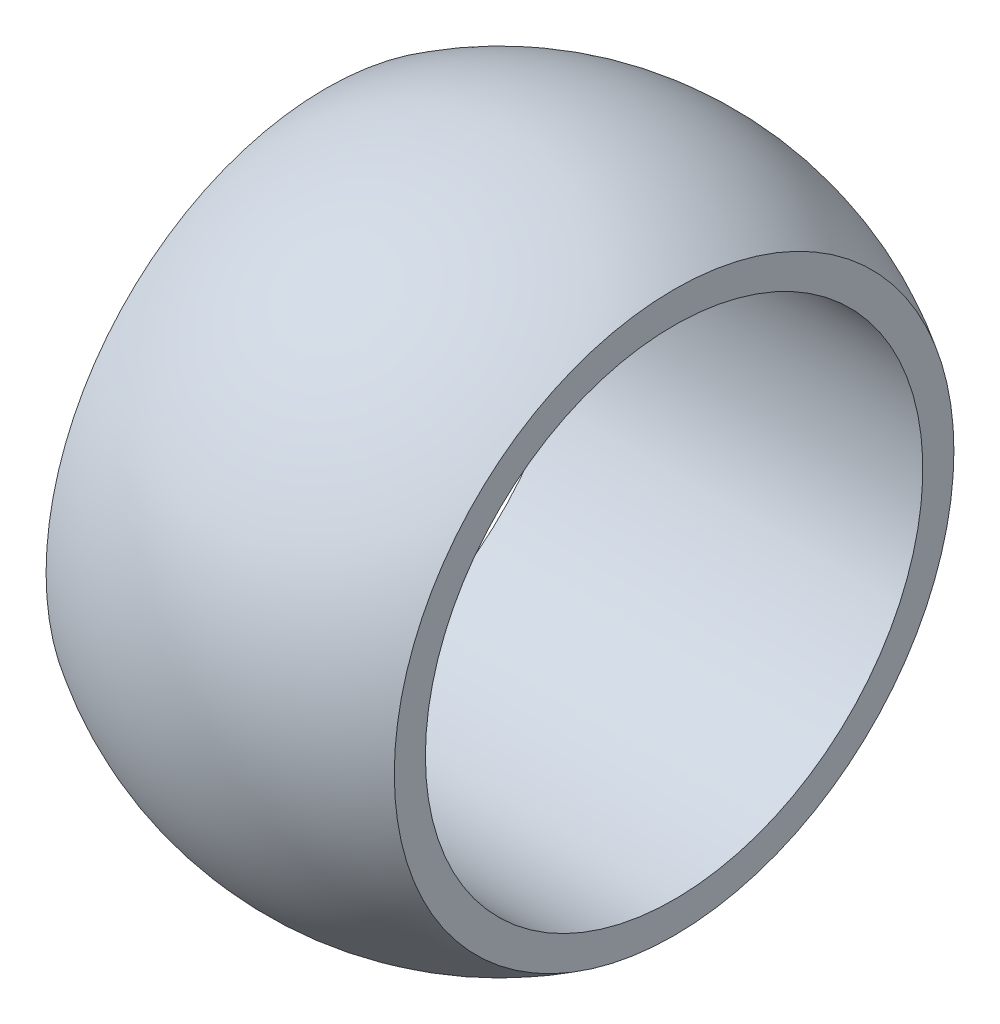
SolidWorks part; units mm, degrees
material "普通碳钢"
ref_plane "前视" through (0, 0, 0) normal (0, 0, 1) x (1, 0, 0)
ref_plane "上视" through (0, 0, 0) normal (0, 1, 0) x (1, 0, 0)
ref_plane "右视" through (0, 0, 0) normal (1, 0, 0) x (0, 0, -1)
sketch "草图1" plane through (0, 0, 0) normal (0, 0, 1) x (1, 0, 0)
  line L0 (-51.7206, 0) -> (61.7182, 0) construction
  line L1 (0, 36.5243) -> (0, -24.6606) construction
  line L2 (-14, 22.5) -> (-14, 20)
  line L3 (14, 22.5) -> (14, 20)
  line L4 (-14, 20) -> (14, 20)
  arc A0 (14, 22.5) -> (-14, 22.5) centre (0, 0) ccw
  dimension "D1" = 53
  dimension "D2" = 28
  dimension "D3" = 20
revolve "旋转1" add sketch "草图1" angle 360 about L0
